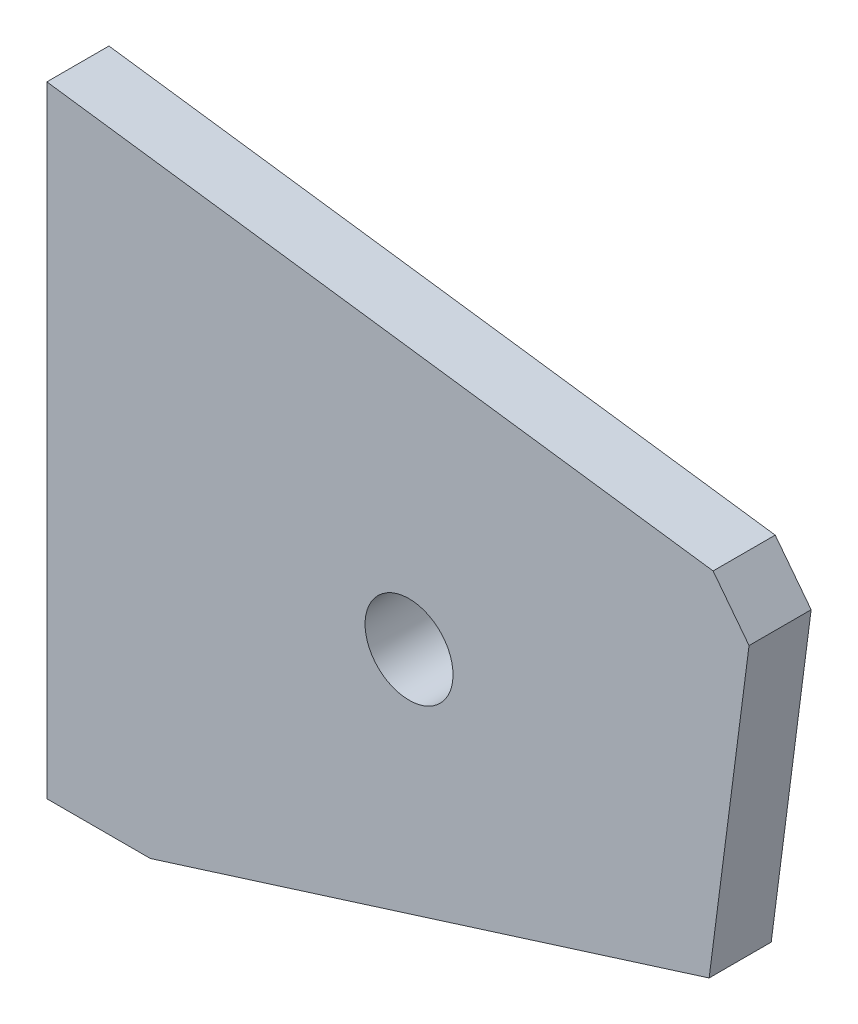
SolidWorks part; units mm, degrees
material "1023 碳钢板 (SS)"
ref_plane "Front Plane" through (0, 0, 0) normal (0, 0, 1) x (1, 0, 0)
ref_plane "Top Plane" through (0, 0, 0) normal (0, 1, 0) x (1, 0, 0)
ref_plane "Right Plane" through (0, 0, 0) normal (1, 0, 0) x (0, 0, -1)
sketch "Sketch1" plane through (0, 0, 0) normal (0, 0, 1) x (1, 0, 0)
  line L0 (0, 0) -> (0, 60)
  line L1 (0, 60) -> (68.3729, 50.7182)
  line L3 (64, 17) -> (10, 0)
  line L4 (10, 0) -> (0, 0)
  line L5 (68.3729, 50.7182) -> (64, 17)
  dimension "D1" = 69
  dimension "D2" = 34
  dimension "D3" = 10
  dimension "D4" = 17
  dimension "D5" = 54
  dimension "D6" = 60
extrude "Boss-Extrude1" add sketch "Sketch1" along normal blind 6 contours L5 L3 L4 L0 L1
sketch "Sketch5" plane through (0, 0, 6) normal (0, 0, 1) x (1, 0, 0)
  line L0 (0, 0) -> (0, 60) construction
  circle A0 centre (35, 30) radius 7.266
  dimension "D1" = 30
  dimension "D2" = 35
hole_wizard "M10 Tapped Hole2" positions "Sketch6" profile "Sketch7" tap size "M10" standard "ISO"
sketch "Sketch6" plane through (0, 0, 6) normal (0, 0, 1) x (1, 0, 0)
  point P0 (35, 30)
sketch "Sketch7" plane through (35, 30, 6) normal (1, 0, 0) x (0, -1, 0)
  line L0 (0, 0) -> (0, 27.0537)
  line L1 (0, 27.0537) -> (4.25, 24.5)
  line L2 (4.25, 24.5) -> (4.25, 0)
  line L5 (4.25, 0) -> (0, 0)
  line L10 (0, 27.0537) -> (-4.25, 24.5) construction
  line L11 (0, -6.35) -> (0, 107.95) construction
  dimension "螺纹孔钻头直径" = 8.5
  dimension "螺纹孔钻头深度" = 24.5
  dimension "导头角度" = 118
cosmetic thread "Hole Thread Line2" parameters "D1"=20, "D2"=10
chamfer "Chamfer1" distance 4 angle 45 1 edges at (68.3729, 50.7182, 3)
